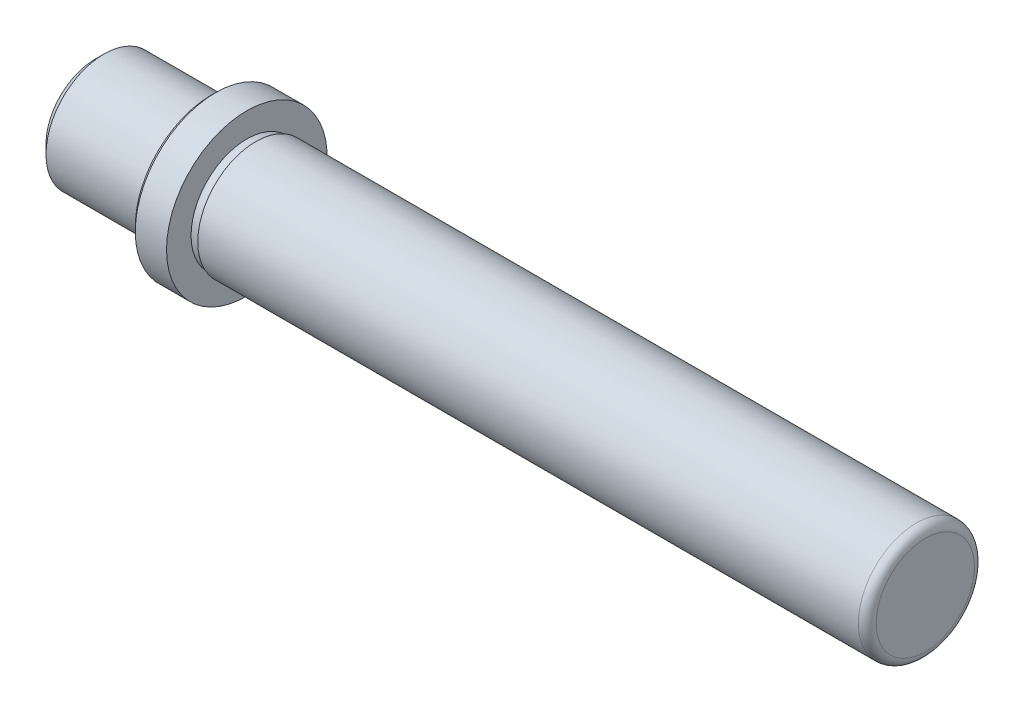
from build123d import *

# Parameters (mm, degrees)
FILLET1_R             = 1
CHAMFER1_SIZE         = 0.5
CHAMFER2_SIZE         = 1
M5_TAPPED_HOLE1_D     = 4.2
M5_TAPPED_HOLE1_DEPTH = 14
M5_TAPPED_HOLE1_TIP   = 1.2618073


with BuildPart() as part:
    # Sketch1 → Revolve1 (revolve)
    with BuildSketch(Plane.XY, mode=Mode.PRIVATE) as revolve1_sk:
        Polygon((13, 6.5), (13, 9), (17, 9), (17, 6.25), (18, 6.25), (18, 6.5), (93, 6.5), (93, 0), (0, 0), (0, 6.5), align=None)
    revolve(revolve1_sk.sketch.rotate(Axis((0, 0, 0), (1, 0, 0)), 90), axis=Axis((0, 0, 0), (1, 0, 0)))

    # Fillet1
    fillet1_edges = [part.edges().sort_by_distance(p)[0] for p in [
        (93, 0, -6.5),
    ]]
    fillet(fillet1_edges, radius=FILLET1_R)

    # Chamfer1
    chamfer1_edges = [part.edges().sort_by_distance(p)[0] for p in [
        (13, 0, -9),
    ]]
    chamfer(chamfer1_edges, length=CHAMFER1_SIZE)

    # Chamfer2
    chamfer2_edges = [part.edges().sort_by_distance(p)[0] for p in [
        (0, 0, -6.5),
    ]]
    chamfer(chamfer2_edges, length=CHAMFER2_SIZE)

    # M5 Tapped Hole1
    with Locations(Plane.ZY):
        with Locations((0, 0)):
            Hole(M5_TAPPED_HOLE1_D / 2, depth=M5_TAPPED_HOLE1_DEPTH)
            with Locations((0, 0, -(M5_TAPPED_HOLE1_DEPTH + M5_TAPPED_HOLE1_TIP / 2))):  # 118° drill point
                Cone(0, M5_TAPPED_HOLE1_D / 2, M5_TAPPED_HOLE1_TIP, mode=Mode.SUBTRACT)


solid = part.part
